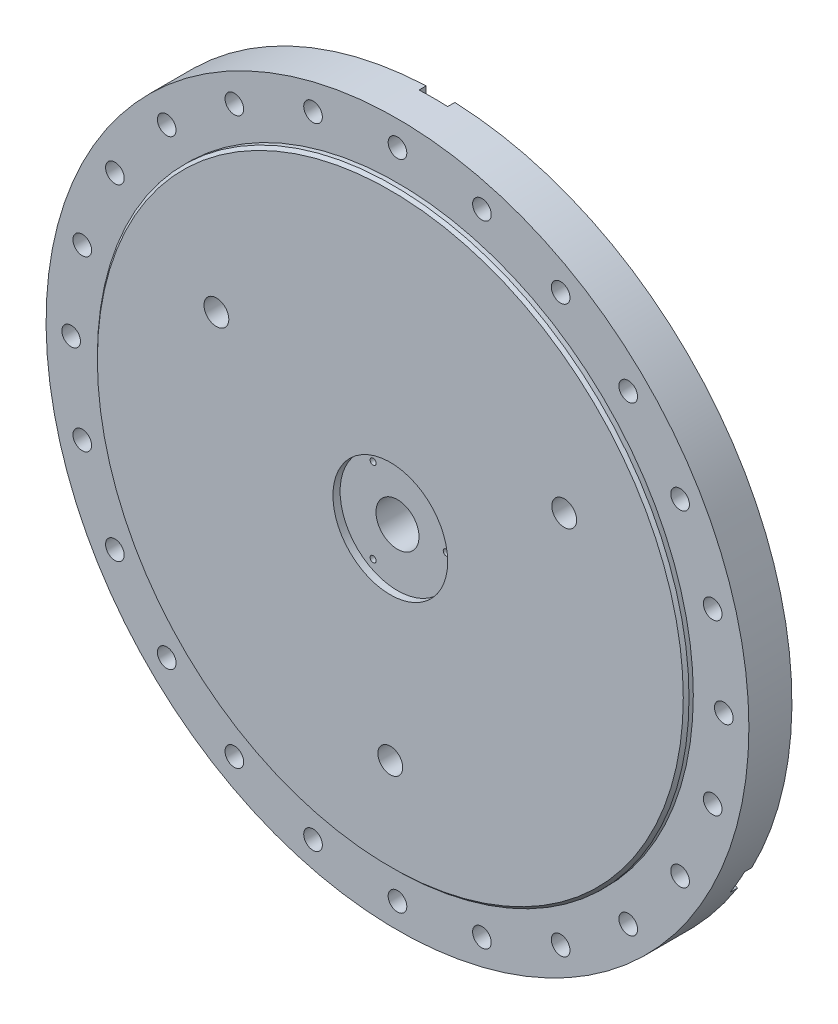
from build123d import *

# Parameters (mm, degrees)
SKETCH1_R                        = 245
BOSS_EXTRUDE2_DEPTH              = 30
SIZE_MM_DOWEL_HOLE_1_AT_2_COUNT  = 2
SIZE_MM_DOWEL_HOLE_1_AT_2_PITCH  = 16
SIZE_MM_DOWEL_HOLE_1_AT_3_COUNT  = 2
SIZE_MM_DOWEL_HOLE_1_AT_3_PITCH  = 32
SIZE_MM_DOWEL_HOLE_1_AT_4_COUNT  = 2
SIZE_MM_DOWEL_HOLE_1_AT_4_PITCH  = 48
SIZE_MM_DOWEL_HOLE_1_AT_5_COUNT  = 2
SIZE_MM_DOWEL_HOLE_1_AT_5_PITCH  = 64
SIZE_MM_DOWEL_HOLE_1_AT_6_COUNT  = 2
SIZE_MM_DOWEL_HOLE_1_AT_6_PITCH  = 80
SIZE_MM_DOWEL_HOLE_1_AT_7_COUNT  = 2
SIZE_MM_DOWEL_HOLE_1_AT_7_PITCH  = 96
SIZE_MM_DOWEL_HOLE_1_AT_8_COUNT  = 2
SIZE_MM_DOWEL_HOLE_1_AT_8_PITCH  = 112
SIZE_MM_DOWEL_HOLE_1_AT_9_COUNT  = 2
SIZE_MM_DOWEL_HOLE_1_AT_9_PITCH  = 128
SIZE_MM_DOWEL_HOLE_1_AT_10_COUNT = 2
SIZE_MM_DOWEL_HOLE_1_AT_10_PITCH = 144
SIZE_MM_DOWEL_HOLE_1_AT_11_COUNT = 2
SIZE_MM_DOWEL_HOLE_1_AT_11_PITCH = 160
SIZE_MM_DOWEL_HOLE_1_AT_12_COUNT = 2
SIZE_MM_DOWEL_HOLE_1_AT_12_PITCH = 176
SIZE_MM_DOWEL_HOLE_1_AT_13_COUNT = 2
SIZE_MM_DOWEL_HOLE_1_AT_13_PITCH = 192
SIZE_MM_DOWEL_HOLE_1_AT_14_COUNT = 2
SIZE_MM_DOWEL_HOLE_1_AT_14_PITCH = 196.968757642
CIRPATTERN2_COUNT                = 3
SIZE_MM_DOWEL_HOLE_4_D           = 4.2
SIZE_MM_DOWEL_HOLE_4_DEPTH       = 14.2
SIZE_MM_DOWEL_HOLE_4_TIP         = 1.2618073
CUT_EXTRUDE1_DEPTH               = 5
CIRPATTERN3_COUNT                = 3
SKETCH7_R                        = 15
CUT_EXTRUDE2_DEPTH               = 352.819396283
MM_4_D                           = 3.2
MM_4_DEPTH                       = 11.8
MM_4_TIP                         = 0.96137699
SKETCH10_R                       = 8.647
SKETCH10_R_2                     = 6.5
CUT_EXTRUDE3_DEPTH               = 353.21000497
SKETCH12_R                       = 10
CUT_EXTRUDE4_DEPTH               = 20
SKETCH13_R                       = 206.25
SKETCH13_R_2                     = 40
SKETCH13_R_3                     = 8.647
BOSS_EXTRUDE3_DEPTH              = 5
MM_4_2_D                         = 4.2
MM_4_2_DEPTH                     = 14.2
MM_4_2_TIP                       = 1.2618073
CHAMFER1_SIZE                    = 2


with BuildPart() as part:
    # Sketch1 → Boss-Extrude2 (new body)
    with BuildSketch(Plane.XY):
        with Locations((-6.250646967, 0)):
            Circle(SKETCH1_R)
    extrude(amount=BOSS_EXTRUDE2_DEPTH)

    # Sketch4 → Size mm Dowel hole 1 (revolve, cut)
    with BuildSketch(Plane(origin=(41.249353033, 228, 0), x_dir=(0, 1, 0), z_dir=(1, 0, 0))):
        Polygon((0, 0), (0, 18.602151548), (2.5, 17.1), (2.5, 0), align=None)
    size_mm_dowel_hole_1 = revolve(axis=Axis((41.249353033, 228, -6.35), (0, 0, 1)), mode=Mode.SUBTRACT)

    # Size mm Dowel hole 1 at 2: Size mm Dowel hole 1 ×2
    with Locations(*[(0, -i * SIZE_MM_DOWEL_HOLE_1_AT_2_PITCH, 0) for i in range(1, SIZE_MM_DOWEL_HOLE_1_AT_2_COUNT)]):
        add(size_mm_dowel_hole_1, mode=Mode.SUBTRACT)

    # Size mm Dowel hole 1 at 3: Size mm Dowel hole 1 ×2
    with Locations(*[(0, -i * SIZE_MM_DOWEL_HOLE_1_AT_3_PITCH, 0) for i in range(1, SIZE_MM_DOWEL_HOLE_1_AT_3_COUNT)]):
        add(size_mm_dowel_hole_1, mode=Mode.SUBTRACT)

    # Size mm Dowel hole 1 at 4: Size mm Dowel hole 1 ×2
    with Locations(*[(0, -i * SIZE_MM_DOWEL_HOLE_1_AT_4_PITCH, 0) for i in range(1, SIZE_MM_DOWEL_HOLE_1_AT_4_COUNT)]):
        add(size_mm_dowel_hole_1, mode=Mode.SUBTRACT)

    # Size mm Dowel hole 1 at 5: Size mm Dowel hole 1 ×2
    with Locations(*[(0, -i * SIZE_MM_DOWEL_HOLE_1_AT_5_PITCH, 0) for i in range(1, SIZE_MM_DOWEL_HOLE_1_AT_5_COUNT)]):
        add(size_mm_dowel_hole_1, mode=Mode.SUBTRACT)

    # Size mm Dowel hole 1 at 6: Size mm Dowel hole 1 ×2
    with Locations(*[(0, -i * SIZE_MM_DOWEL_HOLE_1_AT_6_PITCH, 0) for i in range(1, SIZE_MM_DOWEL_HOLE_1_AT_6_COUNT)]):
        add(size_mm_dowel_hole_1, mode=Mode.SUBTRACT)

    # Size mm Dowel hole 1 at 7: Size mm Dowel hole 1 ×2
    with Locations(*[(0, -i * SIZE_MM_DOWEL_HOLE_1_AT_7_PITCH, 0) for i in range(1, SIZE_MM_DOWEL_HOLE_1_AT_7_COUNT)]):
        add(size_mm_dowel_hole_1, mode=Mode.SUBTRACT)

    # Size mm Dowel hole 1 at 8: Size mm Dowel hole 1 ×2
    with Locations(*[(0, -i * SIZE_MM_DOWEL_HOLE_1_AT_8_PITCH, 0) for i in range(1, SIZE_MM_DOWEL_HOLE_1_AT_8_COUNT)]):
        add(size_mm_dowel_hole_1, mode=Mode.SUBTRACT)

    # Size mm Dowel hole 1 at 9: Size mm Dowel hole 1 ×2
    with Locations(*[(0, -i * SIZE_MM_DOWEL_HOLE_1_AT_9_PITCH, 0) for i in range(1, SIZE_MM_DOWEL_HOLE_1_AT_9_COUNT)]):
        add(size_mm_dowel_hole_1, mode=Mode.SUBTRACT)

    # Size mm Dowel hole 1 at 10: Size mm Dowel hole 1 ×2
    with Locations(*[(0, -i * SIZE_MM_DOWEL_HOLE_1_AT_10_PITCH, 0) for i in range(1, SIZE_MM_DOWEL_HOLE_1_AT_10_COUNT)]):
        add(size_mm_dowel_hole_1, mode=Mode.SUBTRACT)

    # Size mm Dowel hole 1 at 11: Size mm Dowel hole 1 ×2
    with Locations(*[(0, -i * SIZE_MM_DOWEL_HOLE_1_AT_11_PITCH, 0) for i in range(1, SIZE_MM_DOWEL_HOLE_1_AT_11_COUNT)]):
        add(size_mm_dowel_hole_1, mode=Mode.SUBTRACT)

    # Size mm Dowel hole 1 at 12: Size mm Dowel hole 1 ×2
    with Locations(*[(0, -i * SIZE_MM_DOWEL_HOLE_1_AT_12_PITCH, 0) for i in range(1, SIZE_MM_DOWEL_HOLE_1_AT_12_COUNT)]):
        add(size_mm_dowel_hole_1, mode=Mode.SUBTRACT)

    # Size mm Dowel hole 1 at 13: Size mm Dowel hole 1 ×2
    with Locations(*[(0, -i * SIZE_MM_DOWEL_HOLE_1_AT_13_PITCH, 0) for i in range(1, SIZE_MM_DOWEL_HOLE_1_AT_13_COUNT)]):
        add(size_mm_dowel_hole_1, mode=Mode.SUBTRACT)

    # Size mm Dowel hole 1 at 14: Size mm Dowel hole 1 ×2
    with Locations(*[Vector(-0.032642191590678916, -0.9994671016737657, 0) * (i * SIZE_MM_DOWEL_HOLE_1_AT_14_PITCH) for i in range(1, SIZE_MM_DOWEL_HOLE_1_AT_14_COUNT)]):
        add(size_mm_dowel_hole_1, mode=Mode.SUBTRACT)

    # Mirror2: Size mm Dowel hole 1 across plane
    add(size_mm_dowel_hole_1.mirror(Plane.ZY.offset(6.250646967)), mode=Mode.SUBTRACT)

    # Mirror2 copy 1 sketch → Mirror2 copy 1 (revolve, cut)
    with BuildSketch(Plane(origin=(-53.750646967, 212, 0), x_dir=(0, 1, 0), z_dir=(-1, 0, 0))):
        Polygon((0, 0), (0, -18.602151548), (2.5, -17.1), (2.5, 0), align=None)
    revolve(axis=Axis((-53.750646967, 212, -6.35), (0, 0, -1)), mode=Mode.SUBTRACT)

    # Mirror2 copy 2 sketch → Mirror2 copy 2 (revolve, cut)
    with BuildSketch(Plane(origin=(-53.750646967, 196, 0), x_dir=(0, 1, 0), z_dir=(-1, 0, 0))):
        Polygon((0, 0), (0, -18.602151548), (2.5, -17.1), (2.5, 0), align=None)
    revolve(axis=Axis((-53.750646967, 196, -6.35), (0, 0, -1)), mode=Mode.SUBTRACT)

    # Mirror2 copy 3 sketch → Mirror2 copy 3 (revolve, cut)
    with BuildSketch(Plane(origin=(-53.750646967, 180, 0), x_dir=(0, 1, 0), z_dir=(-1, 0, 0))):
        Polygon((0, 0), (0, -18.602151548), (2.5, -17.1), (2.5, 0), align=None)
    revolve(axis=Axis((-53.750646967, 180, -6.35), (0, 0, -1)), mode=Mode.SUBTRACT)

    # Mirror2 copy 4 sketch → Mirror2 copy 4 (revolve, cut)
    with BuildSketch(Plane(origin=(-53.750646967, 164, 0), x_dir=(0, 1, 0), z_dir=(-1, 0, 0))):
        Polygon((0, 0), (0, -18.602151548), (2.5, -17.1), (2.5, 0), align=None)
    revolve(axis=Axis((-53.750646967, 164, -6.35), (0, 0, -1)), mode=Mode.SUBTRACT)

    # Mirror2 copy 5 sketch → Mirror2 copy 5 (revolve, cut)
    with BuildSketch(Plane(origin=(-53.750646967, 148, 0), x_dir=(0, 1, 0), z_dir=(-1, 0, 0))):
        Polygon((0, 0), (0, -18.602151548), (2.5, -17.1), (2.5, 0), align=None)
    revolve(axis=Axis((-53.750646967, 148, -6.35), (0, 0, -1)), mode=Mode.SUBTRACT)

    # Mirror2 copy 6 sketch → Mirror2 copy 6 (revolve, cut)
    with BuildSketch(Plane(origin=(-53.750646967, 132, 0), x_dir=(0, 1, 0), z_dir=(-1, 0, 0))):
        Polygon((0, 0), (0, -18.602151548), (2.5, -17.1), (2.5, 0), align=None)
    revolve(axis=Axis((-53.750646967, 132, -6.35), (0, 0, -1)), mode=Mode.SUBTRACT)

    # Mirror2 copy 7 sketch → Mirror2 copy 7 (revolve, cut)
    with BuildSketch(Plane(origin=(-53.750646967, 116, 0), x_dir=(0, 1, 0), z_dir=(-1, 0, 0))):
        Polygon((0, 0), (0, -18.602151548), (2.5, -17.1), (2.5, 0), align=None)
    revolve(axis=Axis((-53.750646967, 116, -6.35), (0, 0, -1)), mode=Mode.SUBTRACT)

    # Mirror2 copy 8 sketch → Mirror2 copy 8 (revolve, cut)
    with BuildSketch(Plane(origin=(-53.750646967, 100, 0), x_dir=(0, 1, 0), z_dir=(-1, 0, 0))):
        Polygon((0, 0), (0, -18.602151548), (2.5, -17.1), (2.5, 0), align=None)
    revolve(axis=Axis((-53.750646967, 100, -6.35), (0, 0, -1)), mode=Mode.SUBTRACT)

    # Mirror2 copy 9 sketch → Mirror2 copy 9 (revolve, cut)
    with BuildSketch(Plane(origin=(-53.750646967, 84, 0), x_dir=(0, 1, 0), z_dir=(-1, 0, 0))):
        Polygon((0, 0), (0, -18.602151548), (2.5, -17.1), (2.5, 0), align=None)
    revolve(axis=Axis((-53.750646967, 84, -6.35), (0, 0, -1)), mode=Mode.SUBTRACT)

    # Mirror2 copy 10 sketch → Mirror2 copy 10 (revolve, cut)
    with BuildSketch(Plane(origin=(-53.750646967, 68, 0), x_dir=(0, 1, 0), z_dir=(-1, 0, 0))):
        Polygon((0, 0), (0, -18.602151548), (2.5, -17.1), (2.5, 0), align=None)
    revolve(axis=Axis((-53.750646967, 68, -6.35), (0, 0, -1)), mode=Mode.SUBTRACT)

    # Mirror2 copy 11 sketch → Mirror2 copy 11 (revolve, cut)
    with BuildSketch(Plane(origin=(-53.750646967, 52, 0), x_dir=(0, 1, 0), z_dir=(-1, 0, 0))):
        Polygon((0, 0), (0, -18.602151548), (2.5, -17.1), (2.5, 0), align=None)
    revolve(axis=Axis((-53.750646967, 52, -6.35), (0, 0, -1)), mode=Mode.SUBTRACT)

    # Mirror2 copy 12 sketch → Mirror2 copy 12 (revolve, cut)
    with BuildSketch(Plane(origin=(-53.750646967, 36, 0), x_dir=(0, 1, 0), z_dir=(-1, 0, 0))):
        Polygon((0, 0), (0, -18.602151548), (2.5, -17.1), (2.5, 0), align=None)
    revolve(axis=Axis((-53.750646967, 36, -6.35), (0, 0, -1)), mode=Mode.SUBTRACT)

    # Mirror2 copy 13 sketch → Mirror2 copy 13 (revolve, cut)
    with BuildSketch(Plane(origin=(-47.321155042, 31.13620668, 0), x_dir=(0, 1, 0), z_dir=(-1, 0, 0))):
        Polygon((0, 0), (0, -18.602151548), (2.5, -17.1), (2.5, 0), align=None)
    revolve(axis=Axis((-47.321155042, 31.13620668, -6.35), (0, 0, -1)), mode=Mode.SUBTRACT)

    # CirPattern2: Size mm Dowel hole 1 ×3 about axis
    cirpattern2_axis = Axis((-6.250646967, 0, 0), (0, 0, 1))
    for i in range(1, CIRPATTERN2_COUNT):
        add(size_mm_dowel_hole_1.rotate(cirpattern2_axis, i * 360 / CIRPATTERN2_COUNT), mode=Mode.SUBTRACT)

    # CirPattern2 copy 1 sketch → CirPattern2 copy 1 (revolve, cut)
    with BuildSketch(Plane(origin=(-213.598032569, -64.86379332, 0), x_dir=(-0.8660254037844387, -0.4999999999999998, 0), z_dir=(-0.4999999999999998, 0.8660254037844387, 0))):
        Polygon((0, 0), (0, 18.602151548), (2.5, 17.1), (2.5, 0), align=None)
    revolve(axis=Axis((-213.598032569, -64.86379332, -6.35), (0, 0, 1)), mode=Mode.SUBTRACT)

    # CirPattern2 copy 2 sketch → CirPattern2 copy 2 (revolve, cut)
    with BuildSketch(Plane(origin=(153.596738636, -147.13620668, 0), x_dir=(0.8660254037844384, -0.5000000000000004, 0), z_dir=(-0.5000000000000004, -0.8660254037844384, 0))):
        Polygon((0, 0), (0, 18.602151548), (2.5, 17.1), (2.5, 0), align=None)
    revolve(axis=Axis((153.596738636, -147.13620668, -6.35), (0, 0, 1)), mode=Mode.SUBTRACT)

    # CirPattern2 copy 3 sketch → CirPattern2 copy 3 (revolve, cut)
    with BuildSketch(Plane(origin=(-199.741626108, -56.86379332, 0), x_dir=(-0.8660254037844387, -0.4999999999999998, 0), z_dir=(-0.4999999999999998, 0.8660254037844387, 0))):
        Polygon((0, 0), (0, 18.602151548), (2.5, 17.1), (2.5, 0), align=None)
    revolve(axis=Axis((-199.741626108, -56.86379332, -6.35), (0, 0, 1)), mode=Mode.SUBTRACT)

    # CirPattern2 copy 4 sketch → CirPattern2 copy 4 (revolve, cut)
    with BuildSketch(Plane(origin=(139.740332175, -139.13620668, 0), x_dir=(0.8660254037844384, -0.5000000000000004, 0), z_dir=(-0.5000000000000004, -0.8660254037844384, 0))):
        Polygon((0, 0), (0, 18.602151548), (2.5, 17.1), (2.5, 0), align=None)
    revolve(axis=Axis((139.740332175, -139.13620668, -6.35), (0, 0, 1)), mode=Mode.SUBTRACT)

    # CirPattern2 copy 5 sketch → CirPattern2 copy 5 (revolve, cut)
    with BuildSketch(Plane(origin=(-185.885219648, -48.86379332, 0), x_dir=(-0.8660254037844387, -0.4999999999999998, 0), z_dir=(-0.4999999999999998, 0.8660254037844387, 0))):
        Polygon((0, 0), (0, 18.602151548), (2.5, 17.1), (2.5, 0), align=None)
    revolve(axis=Axis((-185.885219648, -48.86379332, -6.35), (0, 0, 1)), mode=Mode.SUBTRACT)

    # CirPattern2 copy 6 sketch → CirPattern2 copy 6 (revolve, cut)
    with BuildSketch(Plane(origin=(125.883925715, -131.13620668, 0), x_dir=(0.8660254037844384, -0.5000000000000004, 0), z_dir=(-0.5000000000000004, -0.8660254037844384, 0))):
        Polygon((0, 0), (0, 18.602151548), (2.5, 17.1), (2.5, 0), align=None)
    revolve(axis=Axis((125.883925715, -131.13620668, -6.35), (0, 0, 1)), mode=Mode.SUBTRACT)

    # CirPattern2 copy 7 sketch → CirPattern2 copy 7 (revolve, cut)
    with BuildSketch(Plane(origin=(-172.028813187, -40.86379332, 0), x_dir=(-0.8660254037844387, -0.4999999999999998, 0), z_dir=(-0.4999999999999998, 0.8660254037844387, 0))):
        Polygon((0, 0), (0, 18.602151548), (2.5, 17.1), (2.5, 0), align=None)
    revolve(axis=Axis((-172.028813187, -40.86379332, -6.35), (0, 0, 1)), mode=Mode.SUBTRACT)

    # CirPattern2 copy 8 sketch → CirPattern2 copy 8 (revolve, cut)
    with BuildSketch(Plane(origin=(112.027519254, -123.13620668, 0), x_dir=(0.8660254037844384, -0.5000000000000004, 0), z_dir=(-0.5000000000000004, -0.8660254037844384, 0))):
        Polygon((0, 0), (0, 18.602151548), (2.5, 17.1), (2.5, 0), align=None)
    revolve(axis=Axis((112.027519254, -123.13620668, -6.35), (0, 0, 1)), mode=Mode.SUBTRACT)

    # CirPattern2 copy 9 sketch → CirPattern2 copy 9 (revolve, cut)
    with BuildSketch(Plane(origin=(-158.172406727, -32.86379332, 0), x_dir=(-0.8660254037844387, -0.4999999999999998, 0), z_dir=(-0.4999999999999998, 0.8660254037844387, 0))):
        Polygon((0, 0), (0, 18.602151548), (2.5, 17.1), (2.5, 0), align=None)
    revolve(axis=Axis((-158.172406727, -32.86379332, -6.35), (0, 0, 1)), mode=Mode.SUBTRACT)

    # CirPattern2 copy 10 sketch → CirPattern2 copy 10 (revolve, cut)
    with BuildSketch(Plane(origin=(98.171112794, -115.13620668, 0), x_dir=(0.8660254037844384, -0.5000000000000004, 0), z_dir=(-0.5000000000000004, -0.8660254037844384, 0))):
        Polygon((0, 0), (0, 18.602151548), (2.5, 17.1), (2.5, 0), align=None)
    revolve(axis=Axis((98.171112794, -115.13620668, -6.35), (0, 0, 1)), mode=Mode.SUBTRACT)

    # CirPattern2 copy 11 sketch → CirPattern2 copy 11 (revolve, cut)
    with BuildSketch(Plane(origin=(-144.316000266, -24.86379332, 0), x_dir=(-0.8660254037844387, -0.4999999999999998, 0), z_dir=(-0.4999999999999998, 0.8660254037844387, 0))):
        Polygon((0, 0), (0, 18.602151548), (2.5, 17.1), (2.5, 0), align=None)
    revolve(axis=Axis((-144.316000266, -24.86379332, -6.35), (0, 0, 1)), mode=Mode.SUBTRACT)

    # CirPattern2 copy 12 sketch → CirPattern2 copy 12 (revolve, cut)
    with BuildSketch(Plane(origin=(84.314706333, -107.13620668, 0), x_dir=(0.8660254037844384, -0.5000000000000004, 0), z_dir=(-0.5000000000000004, -0.8660254037844384, 0))):
        Polygon((0, 0), (0, 18.602151548), (2.5, 17.1), (2.5, 0), align=None)
    revolve(axis=Axis((84.314706333, -107.13620668, -6.35), (0, 0, 1)), mode=Mode.SUBTRACT)

    # CirPattern2 copy 13 sketch → CirPattern2 copy 13 (revolve, cut)
    with BuildSketch(Plane(origin=(-130.459593806, -16.86379332, 0), x_dir=(-0.8660254037844387, -0.4999999999999998, 0), z_dir=(-0.4999999999999998, 0.8660254037844387, 0))):
        Polygon((0, 0), (0, 18.602151548), (2.5, 17.1), (2.5, 0), align=None)
    revolve(axis=Axis((-130.459593806, -16.86379332, -6.35), (0, 0, 1)), mode=Mode.SUBTRACT)

    # CirPattern2 copy 14 sketch → CirPattern2 copy 14 (revolve, cut)
    with BuildSketch(Plane(origin=(70.458299872, -99.13620668, 0), x_dir=(0.8660254037844384, -0.5000000000000004, 0), z_dir=(-0.5000000000000004, -0.8660254037844384, 0))):
        Polygon((0, 0), (0, 18.602151548), (2.5, 17.1), (2.5, 0), align=None)
    revolve(axis=Axis((70.458299872, -99.13620668, -6.35), (0, 0, 1)), mode=Mode.SUBTRACT)

    # CirPattern2 copy 15 sketch → CirPattern2 copy 15 (revolve, cut)
    with BuildSketch(Plane(origin=(-116.603187345, -8.86379332, 0), x_dir=(-0.8660254037844387, -0.4999999999999998, 0), z_dir=(-0.4999999999999998, 0.8660254037844387, 0))):
        Polygon((0, 0), (0, 18.602151548), (2.5, 17.1), (2.5, 0), align=None)
    revolve(axis=Axis((-116.603187345, -8.86379332, -6.35), (0, 0, 1)), mode=Mode.SUBTRACT)

    # CirPattern2 copy 16 sketch → CirPattern2 copy 16 (revolve, cut)
    with BuildSketch(Plane(origin=(56.601893412, -91.13620668, 0), x_dir=(0.8660254037844384, -0.5000000000000004, 0), z_dir=(-0.5000000000000004, -0.8660254037844384, 0))):
        Polygon((0, 0), (0, 18.602151548), (2.5, 17.1), (2.5, 0), align=None)
    revolve(axis=Axis((56.601893412, -91.13620668, -6.35), (0, 0, 1)), mode=Mode.SUBTRACT)

    # CirPattern2 copy 17 sketch → CirPattern2 copy 17 (revolve, cut)
    with BuildSketch(Plane(origin=(-102.746780884, -0.86379332, 0), x_dir=(-0.8660254037844387, -0.4999999999999998, 0), z_dir=(-0.4999999999999998, 0.8660254037844387, 0))):
        Polygon((0, 0), (0, 18.602151548), (2.5, 17.1), (2.5, 0), align=None)
    revolve(axis=Axis((-102.746780884, -0.86379332, -6.35), (0, 0, 1)), mode=Mode.SUBTRACT)

    # CirPattern2 copy 18 sketch → CirPattern2 copy 18 (revolve, cut)
    with BuildSketch(Plane(origin=(42.745486951, -83.13620668, 0), x_dir=(0.8660254037844384, -0.5000000000000004, 0), z_dir=(-0.5000000000000004, -0.8660254037844384, 0))):
        Polygon((0, 0), (0, 18.602151548), (2.5, 17.1), (2.5, 0), align=None)
    revolve(axis=Axis((42.745486951, -83.13620668, -6.35), (0, 0, 1)), mode=Mode.SUBTRACT)

    # CirPattern2 copy 19 sketch → CirPattern2 copy 19 (revolve, cut)
    with BuildSketch(Plane(origin=(-88.890374424, 7.13620668, 0), x_dir=(-0.8660254037844387, -0.4999999999999998, 0), z_dir=(-0.4999999999999998, 0.8660254037844387, 0))):
        Polygon((0, 0), (0, 18.602151548), (2.5, 17.1), (2.5, 0), align=None)
    revolve(axis=Axis((-88.890374424, 7.13620668, -6.35), (0, 0, 1)), mode=Mode.SUBTRACT)

    # CirPattern2 copy 20 sketch → CirPattern2 copy 20 (revolve, cut)
    with BuildSketch(Plane(origin=(28.889080491, -75.13620668, 0), x_dir=(0.8660254037844384, -0.5000000000000004, 0), z_dir=(-0.5000000000000004, -0.8660254037844384, 0))):
        Polygon((0, 0), (0, 18.602151548), (2.5, 17.1), (2.5, 0), align=None)
    revolve(axis=Axis((28.889080491, -75.13620668, -6.35), (0, 0, 1)), mode=Mode.SUBTRACT)

    # CirPattern2 copy 21 sketch → CirPattern2 copy 21 (revolve, cut)
    with BuildSketch(Plane(origin=(-75.033967963, 15.13620668, 0), x_dir=(-0.8660254037844387, -0.4999999999999998, 0), z_dir=(-0.4999999999999998, 0.8660254037844387, 0))):
        Polygon((0, 0), (0, 18.602151548), (2.5, 17.1), (2.5, 0), align=None)
    revolve(axis=Axis((-75.033967963, 15.13620668, -6.35), (0, 0, 1)), mode=Mode.SUBTRACT)

    # CirPattern2 copy 22 sketch → CirPattern2 copy 22 (revolve, cut)
    with BuildSketch(Plane(origin=(15.03267403, -67.13620668, 0), x_dir=(0.8660254037844384, -0.5000000000000004, 0), z_dir=(-0.5000000000000004, -0.8660254037844384, 0))):
        Polygon((0, 0), (0, 18.602151548), (2.5, 17.1), (2.5, 0), align=None)
    revolve(axis=Axis((15.03267403, -67.13620668, -6.35), (0, 0, 1)), mode=Mode.SUBTRACT)

    # CirPattern2 copy 23 sketch → CirPattern2 copy 23 (revolve, cut)
    with BuildSketch(Plane(origin=(-61.177561503, 23.13620668, 0), x_dir=(-0.8660254037844387, -0.4999999999999998, 0), z_dir=(-0.4999999999999998, 0.8660254037844387, 0))):
        Polygon((0, 0), (0, 18.602151548), (2.5, 17.1), (2.5, 0), align=None)
    revolve(axis=Axis((-61.177561503, 23.13620668, -6.35), (0, 0, 1)), mode=Mode.SUBTRACT)

    # CirPattern2 copy 24 sketch → CirPattern2 copy 24 (revolve, cut)
    with BuildSketch(Plane(origin=(1.17626757, -59.13620668, 0), x_dir=(0.8660254037844384, -0.5000000000000004, 0), z_dir=(-0.5000000000000004, -0.8660254037844384, 0))):
        Polygon((0, 0), (0, 18.602151548), (2.5, 17.1), (2.5, 0), align=None)
    revolve(axis=Axis((1.17626757, -59.13620668, -6.35), (0, 0, 1)), mode=Mode.SUBTRACT)

    # CirPattern2 copy 25 sketch → CirPattern2 copy 25 (revolve, cut)
    with BuildSketch(Plane(origin=(-53.750646967, 20, 0), x_dir=(-0.8660254037844387, -0.4999999999999998, 0), z_dir=(-0.4999999999999998, 0.8660254037844387, 0))):
        Polygon((0, 0), (0, 18.602151548), (2.5, 17.1), (2.5, 0), align=None)
    revolve(axis=Axis((-53.750646967, 20, -6.35), (0, 0, 1)), mode=Mode.SUBTRACT)

    # CirPattern2 copy 26 sketch → CirPattern2 copy 26 (revolve, cut)
    with BuildSketch(Plane(origin=(0.178844958, -51.13620668, 0), x_dir=(0.8660254037844384, -0.5000000000000004, 0), z_dir=(-0.5000000000000004, -0.8660254037844384, 0))):
        Polygon((0, 0), (0, 18.602151548), (2.5, 17.1), (2.5, 0), align=None)
    revolve(axis=Axis((0.178844958, -51.13620668, -6.35), (0, 0, 1)), mode=Mode.SUBTRACT)

    # CirPattern2 copy 27 sketch → CirPattern2 copy 27 (revolve, cut)
    with BuildSketch(Plane(origin=(-179.954439029, -155.13620668, 0), x_dir=(-0.8660254037844387, -0.4999999999999998, 0), z_dir=(0.4999999999999998, -0.8660254037844387, 0))):
        Polygon((0, 0), (0, -18.602151548), (2.5, -17.1), (2.5, 0), align=None)
    revolve(axis=Axis((-179.954439029, -155.13620668, -6.35), (0, 0, -1)), mode=Mode.SUBTRACT)

    # CirPattern2 copy 28 sketch → CirPattern2 copy 28 (revolve, cut)
    with BuildSketch(Plane(origin=(214.953145096, -72.86379332, 0), x_dir=(0.8660254037844384, -0.5000000000000004, 0), z_dir=(0.5000000000000004, 0.8660254037844384, 0))):
        Polygon((0, 0), (0, -18.602151548), (2.5, -17.1), (2.5, 0), align=None)
    revolve(axis=Axis((214.953145096, -72.86379332, -6.35), (0, 0, -1)), mode=Mode.SUBTRACT)

    # CirPattern2 copy 29 sketch → CirPattern2 copy 29 (revolve, cut)
    with BuildSketch(Plane(origin=(-166.098032569, -147.13620668, 0), x_dir=(-0.8660254037844387, -0.4999999999999998, 0), z_dir=(0.4999999999999998, -0.8660254037844387, 0))):
        Polygon((0, 0), (0, -18.602151548), (2.5, -17.1), (2.5, 0), align=None)
    revolve(axis=Axis((-166.098032569, -147.13620668, -6.35), (0, 0, -1)), mode=Mode.SUBTRACT)

    # CirPattern2 copy 30 sketch → CirPattern2 copy 30 (revolve, cut)
    with BuildSketch(Plane(origin=(201.096738636, -64.86379332, 0), x_dir=(0.8660254037844384, -0.5000000000000004, 0), z_dir=(0.5000000000000004, 0.8660254037844384, 0))):
        Polygon((0, 0), (0, -18.602151548), (2.5, -17.1), (2.5, 0), align=None)
    revolve(axis=Axis((201.096738636, -64.86379332, -6.35), (0, 0, -1)), mode=Mode.SUBTRACT)

    # CirPattern2 copy 31 sketch → CirPattern2 copy 31 (revolve, cut)
    with BuildSketch(Plane(origin=(-152.241626108, -139.13620668, 0), x_dir=(-0.8660254037844387, -0.4999999999999998, 0), z_dir=(0.4999999999999998, -0.8660254037844387, 0))):
        Polygon((0, 0), (0, -18.602151548), (2.5, -17.1), (2.5, 0), align=None)
    revolve(axis=Axis((-152.241626108, -139.13620668, -6.35), (0, 0, -1)), mode=Mode.SUBTRACT)

    # CirPattern2 copy 32 sketch → CirPattern2 copy 32 (revolve, cut)
    with BuildSketch(Plane(origin=(187.240332175, -56.86379332, 0), x_dir=(0.8660254037844384, -0.5000000000000004, 0), z_dir=(0.5000000000000004, 0.8660254037844384, 0))):
        Polygon((0, 0), (0, -18.602151548), (2.5, -17.1), (2.5, 0), align=None)
    revolve(axis=Axis((187.240332175, -56.86379332, -6.35), (0, 0, -1)), mode=Mode.SUBTRACT)

    # CirPattern2 copy 33 sketch → CirPattern2 copy 33 (revolve, cut)
    with BuildSketch(Plane(origin=(-138.385219648, -131.13620668, 0), x_dir=(-0.8660254037844387, -0.4999999999999998, 0), z_dir=(0.4999999999999998, -0.8660254037844387, 0))):
        Polygon((0, 0), (0, -18.602151548), (2.5, -17.1), (2.5, 0), align=None)
    revolve(axis=Axis((-138.385219648, -131.13620668, -6.35), (0, 0, -1)), mode=Mode.SUBTRACT)

    # CirPattern2 copy 34 sketch → CirPattern2 copy 34 (revolve, cut)
    with BuildSketch(Plane(origin=(173.383925715, -48.86379332, 0), x_dir=(0.8660254037844384, -0.5000000000000004, 0), z_dir=(0.5000000000000004, 0.8660254037844384, 0))):
        Polygon((0, 0), (0, -18.602151548), (2.5, -17.1), (2.5, 0), align=None)
    revolve(axis=Axis((173.383925715, -48.86379332, -6.35), (0, 0, -1)), mode=Mode.SUBTRACT)

    # CirPattern2 copy 35 sketch → CirPattern2 copy 35 (revolve, cut)
    with BuildSketch(Plane(origin=(-124.528813187, -123.13620668, 0), x_dir=(-0.8660254037844387, -0.4999999999999998, 0), z_dir=(0.4999999999999998, -0.8660254037844387, 0))):
        Polygon((0, 0), (0, -18.602151548), (2.5, -17.1), (2.5, 0), align=None)
    revolve(axis=Axis((-124.528813187, -123.13620668, -6.35), (0, 0, -1)), mode=Mode.SUBTRACT)

    # CirPattern2 copy 36 sketch → CirPattern2 copy 36 (revolve, cut)
    with BuildSketch(Plane(origin=(159.527519254, -40.86379332, 0), x_dir=(0.8660254037844384, -0.5000000000000004, 0), z_dir=(0.5000000000000004, 0.8660254037844384, 0))):
        Polygon((0, 0), (0, -18.602151548), (2.5, -17.1), (2.5, 0), align=None)
    revolve(axis=Axis((159.527519254, -40.86379332, -6.35), (0, 0, -1)), mode=Mode.SUBTRACT)

    # CirPattern2 copy 37 sketch → CirPattern2 copy 37 (revolve, cut)
    with BuildSketch(Plane(origin=(-110.672406727, -115.13620668, 0), x_dir=(-0.8660254037844387, -0.4999999999999998, 0), z_dir=(0.4999999999999998, -0.8660254037844387, 0))):
        Polygon((0, 0), (0, -18.602151548), (2.5, -17.1), (2.5, 0), align=None)
    revolve(axis=Axis((-110.672406727, -115.13620668, -6.35), (0, 0, -1)), mode=Mode.SUBTRACT)

    # CirPattern2 copy 38 sketch → CirPattern2 copy 38 (revolve, cut)
    with BuildSketch(Plane(origin=(145.671112794, -32.86379332, 0), x_dir=(0.8660254037844384, -0.5000000000000004, 0), z_dir=(0.5000000000000004, 0.8660254037844384, 0))):
        Polygon((0, 0), (0, -18.602151548), (2.5, -17.1), (2.5, 0), align=None)
    revolve(axis=Axis((145.671112794, -32.86379332, -6.35), (0, 0, -1)), mode=Mode.SUBTRACT)

    # CirPattern2 copy 39 sketch → CirPattern2 copy 39 (revolve, cut)
    with BuildSketch(Plane(origin=(-96.816000266, -107.13620668, 0), x_dir=(-0.8660254037844387, -0.4999999999999998, 0), z_dir=(0.4999999999999998, -0.8660254037844387, 0))):
        Polygon((0, 0), (0, -18.602151548), (2.5, -17.1), (2.5, 0), align=None)
    revolve(axis=Axis((-96.816000266, -107.13620668, -6.35), (0, 0, -1)), mode=Mode.SUBTRACT)

    # CirPattern2 copy 40 sketch → CirPattern2 copy 40 (revolve, cut)
    with BuildSketch(Plane(origin=(131.814706333, -24.86379332, 0), x_dir=(0.8660254037844384, -0.5000000000000004, 0), z_dir=(0.5000000000000004, 0.8660254037844384, 0))):
        Polygon((0, 0), (0, -18.602151548), (2.5, -17.1), (2.5, 0), align=None)
    revolve(axis=Axis((131.814706333, -24.86379332, -6.35), (0, 0, -1)), mode=Mode.SUBTRACT)

    # CirPattern2 copy 41 sketch → CirPattern2 copy 41 (revolve, cut)
    with BuildSketch(Plane(origin=(-82.959593806, -99.13620668, 0), x_dir=(-0.8660254037844387, -0.4999999999999998, 0), z_dir=(0.4999999999999998, -0.8660254037844387, 0))):
        Polygon((0, 0), (0, -18.602151548), (2.5, -17.1), (2.5, 0), align=None)
    revolve(axis=Axis((-82.959593806, -99.13620668, -6.35), (0, 0, -1)), mode=Mode.SUBTRACT)

    # CirPattern2 copy 42 sketch → CirPattern2 copy 42 (revolve, cut)
    with BuildSketch(Plane(origin=(117.958299872, -16.86379332, 0), x_dir=(0.8660254037844384, -0.5000000000000004, 0), z_dir=(0.5000000000000004, 0.8660254037844384, 0))):
        Polygon((0, 0), (0, -18.602151548), (2.5, -17.1), (2.5, 0), align=None)
    revolve(axis=Axis((117.958299872, -16.86379332, -6.35), (0, 0, -1)), mode=Mode.SUBTRACT)

    # CirPattern2 copy 43 sketch → CirPattern2 copy 43 (revolve, cut)
    with BuildSketch(Plane(origin=(-69.103187345, -91.13620668, 0), x_dir=(-0.8660254037844387, -0.4999999999999998, 0), z_dir=(0.4999999999999998, -0.8660254037844387, 0))):
        Polygon((0, 0), (0, -18.602151548), (2.5, -17.1), (2.5, 0), align=None)
    revolve(axis=Axis((-69.103187345, -91.13620668, -6.35), (0, 0, -1)), mode=Mode.SUBTRACT)

    # CirPattern2 copy 44 sketch → CirPattern2 copy 44 (revolve, cut)
    with BuildSketch(Plane(origin=(104.101893412, -8.86379332, 0), x_dir=(0.8660254037844384, -0.5000000000000004, 0), z_dir=(0.5000000000000004, 0.8660254037844384, 0))):
        Polygon((0, 0), (0, -18.602151548), (2.5, -17.1), (2.5, 0), align=None)
    revolve(axis=Axis((104.101893412, -8.86379332, -6.35), (0, 0, -1)), mode=Mode.SUBTRACT)

    # CirPattern2 copy 45 sketch → CirPattern2 copy 45 (revolve, cut)
    with BuildSketch(Plane(origin=(-55.246780884, -83.13620668, 0), x_dir=(-0.8660254037844387, -0.4999999999999998, 0), z_dir=(0.4999999999999998, -0.8660254037844387, 0))):
        Polygon((0, 0), (0, -18.602151548), (2.5, -17.1), (2.5, 0), align=None)
    revolve(axis=Axis((-55.246780884, -83.13620668, -6.35), (0, 0, -1)), mode=Mode.SUBTRACT)

    # CirPattern2 copy 46 sketch → CirPattern2 copy 46 (revolve, cut)
    with BuildSketch(Plane(origin=(90.245486951, -0.86379332, 0), x_dir=(0.8660254037844384, -0.5000000000000004, 0), z_dir=(0.5000000000000004, 0.8660254037844384, 0))):
        Polygon((0, 0), (0, -18.602151548), (2.5, -17.1), (2.5, 0), align=None)
    revolve(axis=Axis((90.245486951, -0.86379332, -6.35), (0, 0, -1)), mode=Mode.SUBTRACT)

    # CirPattern2 copy 47 sketch → CirPattern2 copy 47 (revolve, cut)
    with BuildSketch(Plane(origin=(-41.390374424, -75.13620668, 0), x_dir=(-0.8660254037844387, -0.4999999999999998, 0), z_dir=(0.4999999999999998, -0.8660254037844387, 0))):
        Polygon((0, 0), (0, -18.602151548), (2.5, -17.1), (2.5, 0), align=None)
    revolve(axis=Axis((-41.390374424, -75.13620668, -6.35), (0, 0, -1)), mode=Mode.SUBTRACT)

    # CirPattern2 copy 48 sketch → CirPattern2 copy 48 (revolve, cut)
    with BuildSketch(Plane(origin=(76.389080491, 7.13620668, 0), x_dir=(0.8660254037844384, -0.5000000000000004, 0), z_dir=(0.5000000000000004, 0.8660254037844384, 0))):
        Polygon((0, 0), (0, -18.602151548), (2.5, -17.1), (2.5, 0), align=None)
    revolve(axis=Axis((76.389080491, 7.13620668, -6.35), (0, 0, -1)), mode=Mode.SUBTRACT)

    # CirPattern2 copy 49 sketch → CirPattern2 copy 49 (revolve, cut)
    with BuildSketch(Plane(origin=(-27.533967963, -67.13620668, 0), x_dir=(-0.8660254037844387, -0.4999999999999998, 0), z_dir=(0.4999999999999998, -0.8660254037844387, 0))):
        Polygon((0, 0), (0, -18.602151548), (2.5, -17.1), (2.5, 0), align=None)
    revolve(axis=Axis((-27.533967963, -67.13620668, -6.35), (0, 0, -1)), mode=Mode.SUBTRACT)

    # CirPattern2 copy 50 sketch → CirPattern2 copy 50 (revolve, cut)
    with BuildSketch(Plane(origin=(62.53267403, 15.13620668, 0), x_dir=(0.8660254037844384, -0.5000000000000004, 0), z_dir=(0.5000000000000004, 0.8660254037844384, 0))):
        Polygon((0, 0), (0, -18.602151548), (2.5, -17.1), (2.5, 0), align=None)
    revolve(axis=Axis((62.53267403, 15.13620668, -6.35), (0, 0, -1)), mode=Mode.SUBTRACT)

    # CirPattern2 copy 51 sketch → CirPattern2 copy 51 (revolve, cut)
    with BuildSketch(Plane(origin=(-13.677561503, -59.13620668, 0), x_dir=(-0.8660254037844387, -0.4999999999999998, 0), z_dir=(0.4999999999999998, -0.8660254037844387, 0))):
        Polygon((0, 0), (0, -18.602151548), (2.5, -17.1), (2.5, 0), align=None)
    revolve(axis=Axis((-13.677561503, -59.13620668, -6.35), (0, 0, -1)), mode=Mode.SUBTRACT)

    # CirPattern2 copy 52 sketch → CirPattern2 copy 52 (revolve, cut)
    with BuildSketch(Plane(origin=(48.67626757, 23.13620668, 0), x_dir=(0.8660254037844384, -0.5000000000000004, 0), z_dir=(0.5000000000000004, 0.8660254037844384, 0))):
        Polygon((0, 0), (0, -18.602151548), (2.5, -17.1), (2.5, 0), align=None)
    revolve(axis=Axis((48.67626757, 23.13620668, -6.35), (0, 0, -1)), mode=Mode.SUBTRACT)

    # CirPattern2 copy 53 sketch → CirPattern2 copy 53 (revolve, cut)
    with BuildSketch(Plane(origin=(-12.680138891, -51.13620668, 0), x_dir=(-0.8660254037844387, -0.4999999999999998, 0), z_dir=(0.4999999999999998, -0.8660254037844387, 0))):
        Polygon((0, 0), (0, -18.602151548), (2.5, -17.1), (2.5, 0), align=None)
    revolve(axis=Axis((-12.680138891, -51.13620668, -6.35), (0, 0, -1)), mode=Mode.SUBTRACT)

    # CirPattern2 copy 54 sketch → CirPattern2 copy 54 (revolve, cut)
    with BuildSketch(Plane(origin=(41.249353033, 20, 0), x_dir=(0.8660254037844384, -0.5000000000000004, 0), z_dir=(0.5000000000000004, 0.8660254037844384, 0))):
        Polygon((0, 0), (0, -18.602151548), (2.5, -17.1), (2.5, 0), align=None)
    revolve(axis=Axis((41.249353033, 20, -6.35), (0, 0, -1)), mode=Mode.SUBTRACT)

    # Size mm Dowel hole 4
    with Locations(Plane(origin=(0, 0, 0), x_dir=(-1, 0, 0), z_dir=(0, 0, -1))):
        with Locations((-13.749353033, 235), (26.250646967, 235), (219.766616856, -100.179491924), (199.766616856, -134.820508076), (-207.265322923, -100.179491924), (-187.265322923, -134.820508076)):
            Hole(SIZE_MM_DOWEL_HOLE_4_D / 2, depth=SIZE_MM_DOWEL_HOLE_4_DEPTH)
            with Locations((0, 0, -(SIZE_MM_DOWEL_HOLE_4_DEPTH + SIZE_MM_DOWEL_HOLE_4_TIP / 2))):  # 118° drill point
                Cone(0, SIZE_MM_DOWEL_HOLE_4_D / 2, SIZE_MM_DOWEL_HOLE_4_TIP, mode=Mode.SUBTRACT)

    # Sketch6 → Cut-Extrude1 (cut)
    with BuildSketch(Plane(origin=(0, 0, 0), x_dir=(-1, 0, 0), z_dir=(0, 0, -1))):
        with BuildLine():
            Line((-3.749353033, -45), (16.250646967, -45))
            Line((16.250646967, -45), (16.250646967, -17.320508076))
            ThreePointArc((16.250646967, -17.320508076), (26.250646967, 0), (16.250646967, 17.320508076))
            Line((16.250646967, 17.320508076), (16.250646967, 297.970403072))
            Line((16.250646967, 297.970403072), (-3.749353033, 297.970403072))
            Line((-3.749353033, 297.970403072), (-3.749353033, 17.320508076))
            ThreePointArc((-3.749353033, 17.320508076), (-13.749353033, 0), (-3.749353033, -17.320508076))
            Line((-3.749353033, -17.320508076), (-3.749353033, -45))
        make_face()
    cut_extrude1 = extrude(amount=-CUT_EXTRUDE1_DEPTH, mode=Mode.SUBTRACT)

    # CirPattern3: Cut-Extrude1 ×3 about axis
    cirpattern3_axis = Axis((-6.250646967, 0, 0), (0, 0, 1))
    for i in range(1, CIRPATTERN3_COUNT):
        add(cut_extrude1.rotate(cirpattern3_axis, i * 360 / CIRPATTERN3_COUNT), mode=Mode.SUBTRACT)

    # Sketch7 → Cut-Extrude2 (cut, through all)
    with BuildSketch(Plane(origin=(0, 0, 5), x_dir=(-1, 0, 0), z_dir=(0, 0, -1))):
        with Locations((6.250646967, 0)):
            Circle(SKETCH7_R)
    extrude(amount=-CUT_EXTRUDE2_DEPTH, mode=Mode.SUBTRACT)

    # mm _4
    with Locations(Plane(origin=(0, 0, 0), x_dir=(-1, 0, 0), z_dir=(0, 0, -1))):
        with Locations((-97.492909563, 100.310889132), (-132.492909563, 39.689110868), (109.994203496, 100.310889132), (144.994203496, 39.689110868), (41.250646967, -140), (-28.749353033, -140)):
            Hole(MM_4_D / 2, depth=MM_4_DEPTH)
            with Locations((0, 0, -(MM_4_DEPTH + MM_4_TIP / 2))):  # 118° drill point
                Cone(0, MM_4_D / 2, MM_4_TIP, mode=Mode.SUBTRACT)

    # Sketch10 → Cut-Extrude3 (cut, through all)
    with BuildSketch(Plane(origin=(0, 0, 0), x_dir=(-1, 0, 0), z_dir=(0, 0, -1))):
        with Locations((-114.992909563, 70)):
            Circle(SKETCH10_R)
        with Locations((127.494203496, 70)):
            Circle(SKETCH10_R)
        with Locations((6.250646967, -140)):
            Circle(SKETCH10_R)
        with Locations((-190.770132394, 113.75)):
            Circle(SKETCH10_R_2)
        with Locations((-154.616145753, 160.86679272)):
            Circle(SKETCH10_R_2)
        with Locations((-107.499353033, 197.020779361)):
            Circle(SKETCH10_R_2)
        with Locations((-52.630685794, 219.748125481)):
            Circle(SKETCH10_R_2)
        with Locations((6.250646967, 227.5)):
            Circle(SKETCH10_R_2)
        with Locations((65.131979727, 219.748125481)):
            Circle(SKETCH10_R_2)
        with Locations((120.000646967, 197.020779361)):
            Circle(SKETCH10_R_2)
        with Locations((167.117439687, 160.86679272)):
            Circle(SKETCH10_R_2)
        with Locations((203.271426328, 113.75)):
            Circle(SKETCH10_R_2)
        with Locations((225.998772447, 58.881332761)):
            Circle(SKETCH10_R_2)
        with Locations((233.750646967, 0)):
            Circle(SKETCH10_R_2)
        with Locations((225.998772447, -58.881332761)):
            Circle(SKETCH10_R_2)
        with Locations((203.271426328, -113.75)):
            Circle(SKETCH10_R_2)
        with Locations((167.117439687, -160.86679272)):
            Circle(SKETCH10_R_2)
        with Locations((120.000646967, -197.020779361)):
            Circle(SKETCH10_R_2)
        with Locations((65.131979727, -219.748125481)):
            Circle(SKETCH10_R_2)
        with Locations((6.250646967, -227.5)):
            Circle(SKETCH10_R_2)
        with Locations((-52.630685794, -219.748125481)):
            Circle(SKETCH10_R_2)
        with Locations((-107.499353033, -197.020779361)):
            Circle(SKETCH10_R_2)
        with Locations((-154.616145753, -160.86679272)):
            Circle(SKETCH10_R_2)
        with Locations((-190.770132394, -113.75)):
            Circle(SKETCH10_R_2)
        with Locations((-213.497478514, -58.881332761)):
            Circle(SKETCH10_R_2)
        with Locations((-221.249353033, 0)):
            Circle(SKETCH10_R_2)
        with Locations((-213.497478514, 58.881332761)):
            Circle(SKETCH10_R_2)
    extrude(amount=-CUT_EXTRUDE3_DEPTH, mode=Mode.SUBTRACT)

    # Sketch12 → Cut-Extrude4 (cut)
    with BuildSketch(Plane(origin=(0, 0, 0), x_dir=(-1, 0, 0), z_dir=(0, 0, -1))):
        with Locations((-154.616145753, 160.86679272)):
            Circle(SKETCH12_R)
        with Locations((-107.499353033, 197.020779361)):
            Circle(SKETCH12_R)
        with Locations((-52.630685794, 219.748125481)):
            Circle(SKETCH12_R)
        with Locations((6.250646967, 227.5)):
            Circle(SKETCH12_R)
        with Locations((65.131979727, 219.748125481)):
            Circle(SKETCH12_R)
        with Locations((120.000646967, 197.020779361)):
            Circle(SKETCH12_R)
        with Locations((167.117439687, 160.86679272)):
            Circle(SKETCH12_R)
        with Locations((203.271426328, 113.75)):
            Circle(SKETCH12_R)
        with Locations((225.998772447, 58.881332761)):
            Circle(SKETCH12_R)
        with Locations((233.750646967, 0)):
            Circle(SKETCH12_R)
        with Locations((225.998772447, -58.881332761)):
            Circle(SKETCH12_R)
        with Locations((203.271426328, -113.75)):
            Circle(SKETCH12_R)
        with Locations((167.117439687, -160.86679272)):
            Circle(SKETCH12_R)
        with Locations((120.000646967, -197.020779361)):
            Circle(SKETCH12_R)
        with Locations((65.131979727, -219.748125481)):
            Circle(SKETCH12_R)
        with Locations((6.250646967, -227.5)):
            Circle(SKETCH12_R)
        with Locations((-52.630685794, -219.748125481)):
            Circle(SKETCH12_R)
        with Locations((-107.499353033, -197.020779361)):
            Circle(SKETCH12_R)
        with Locations((-154.616145753, -160.86679272)):
            Circle(SKETCH12_R)
        with Locations((-190.770132394, -113.75)):
            Circle(SKETCH12_R)
        with Locations((-213.497478514, -58.881332761)):
            Circle(SKETCH12_R)
        with Locations((-221.249353033, 0)):
            Circle(SKETCH12_R)
        with Locations((-213.497478514, 58.881332761)):
            Circle(SKETCH12_R)
        with Locations((-190.770132394, 113.75)):
            Circle(SKETCH12_R)
    extrude(amount=-CUT_EXTRUDE4_DEPTH, mode=Mode.SUBTRACT)

    # Sketch13 → Boss-Extrude3 (add)
    with BuildSketch(Plane.XY.offset(30)):
        with Locations((-6.250646967, 0)):
            Circle(SKETCH13_R)
        with Locations((-6.250646967, 0)):
            Circle(SKETCH13_R_2, mode=Mode.SUBTRACT)
        with Locations(Location((-127.494203496, 70, 0), (0, 0, 180))):
            Circle(SKETCH13_R_3, mode=Mode.SUBTRACT)
        with Locations(Location((114.992909563, 70, 0), (0, 0, 180))):
            Circle(SKETCH13_R_3, mode=Mode.SUBTRACT)
        with Locations(Location((-6.250646967, -140, 0), (0, 0, 180))):
            Circle(SKETCH13_R_3, mode=Mode.SUBTRACT)
    extrude(amount=BOSS_EXTRUDE3_DEPTH)

    # mm _4 2
    with Locations(Plane.XY.offset(35)):
        with Locations((-23.250646967, 29.444863729), (-23.250646967, -29.444863729), (27.749353033, 0)):
            Hole(MM_4_2_D / 2, depth=MM_4_2_DEPTH)
            with Locations((0, 0, -(MM_4_2_DEPTH + MM_4_2_TIP / 2))):  # 118° drill point
                Cone(0, MM_4_2_D / 2, MM_4_2_TIP, mode=Mode.SUBTRACT)

    # Chamfer1
    chamfer1_edges = [part.edges().sort_by_distance(p)[0] for p in [
        (-212.500646967, 0, 35),
    ]]
    chamfer(chamfer1_edges, length=CHAMFER1_SIZE)


solid = part.part
